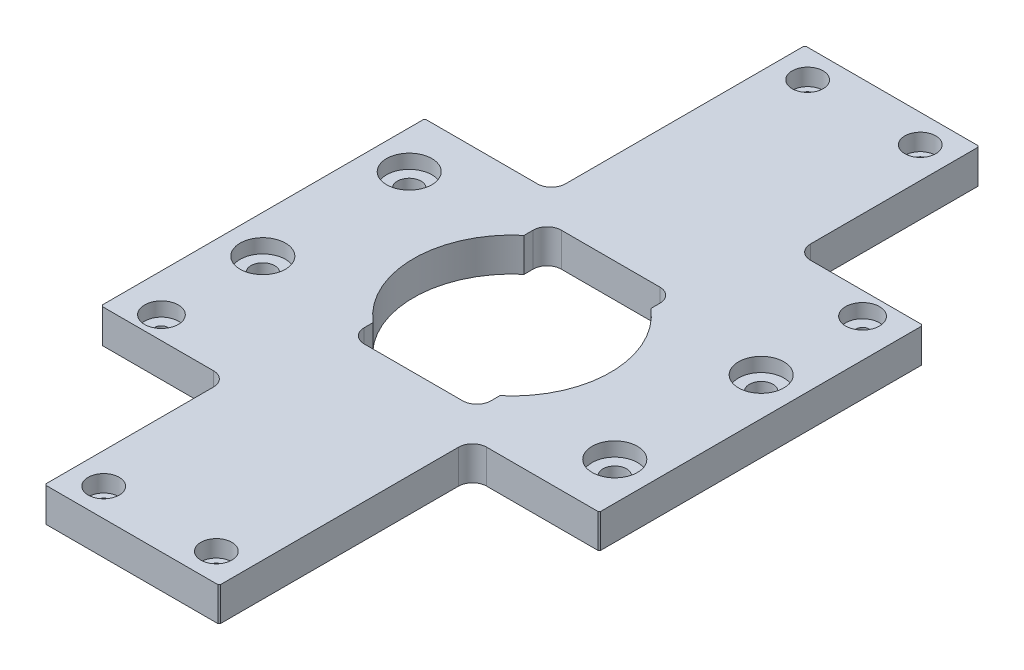
SolidWorks part; units mm, degrees
material "AL6061"
ref_plane "Front Plane" through (0, 0, 0) normal (0, 0, 1) x (1, 0, 0)
ref_plane "Top Plane" through (0, 0, 0) normal (0, 1, 0) x (1, 0, 0)
ref_plane "Right Plane" through (0, 0, 0) normal (1, 0, 0) x (0, 0, -1)
sketch "Sketch1" plane through (0, 0, 0) normal (0, 1, 0) x (1, 0, 0)
  line L1 (-76, -135) -> (76, -135)
  line L2 (-76, -135) -> (-76, 135)
  line L3 (-76, 135) -> (76, 135)
  line L4 (76, -135) -> (76, 135)
  line L5 (-76, -135) -> (76, 135) construction
  line L6 (-76, 135) -> (76, -135) construction
  point P0 (0, 0)
  dimension "D1" = 152
  dimension "D2" = 270
extrude "Boss-Extrude1" add sketch "Sketch1" along normal mid plane 12
sketch "Sketch2" plane through (0, 6, 0) normal (0, 1, 0) x (1, 0, 0)
  circle A0 centre (0, 0) radius 35
  dimension "D1" = 70
extrude "Cut-Extrude1" cut sketch "Sketch2" against normal through all
sketch "Sketch5" plane through (0, 6, 0) normal (0, 1, 0) x (1, 0, 0)
  line L0 (0, 0) -> (-109.7295, 0) construction
  line L1 (0, 0) -> (0, 145.3543) construction
  line L2 (62.5, 62) -> (62.5, -123.0833) construction
  circle A0 centre (62.5, 62) radius 6
  circle A1 centre (-62.5, 62) radius 6 construction
  circle A2 centre (-62.5, -62) radius 6
  circle A3 centre (62.5, -62) radius 6 construction
  circle A4 centre (62.5, 26) radius 8.05
  circle A5 centre (-62.5, 26) radius 8.05
  circle A6 centre (-62.5, -26) radius 8.05
  circle A7 centre (62.5, -26) radius 8.05
  dimension "D1" = 124
  dimension "D2" = 125
  dimension "D3" = 12
  dimension "D4" = 16.1
  dimension "D5" = 52
extrude "Cut-Extrude2" cut sketch "Sketch5" against normal blind 5
sketch "Sketch6" plane through (0, 6, 0) normal (0, 1, 0) x (1, 0, 0)
  line L1 (-22.5, -35) -> (22.5, -35)
  line L2 (-22.5, -35) -> (-22.5, 35)
  line L3 (-22.5, 35) -> (22.5, 35)
  line L4 (22.5, -35) -> (22.5, 35)
  line L5 (-22.5, -35) -> (22.5, 35) construction
  line L6 (-22.5, 35) -> (22.5, -35) construction
  point P0 (0, 0)
  dimension "D1" = 70
  dimension "D2" = 45
extrude "Cut-Extrude3" cut sketch "Sketch6" against normal through all
sketch "Sketch7" plane through (0, 6, 0) normal (0, 1, 0) x (1, 0, 0)
  line L0 (0, 0) -> (0, 159.161) construction
  line L1 (0, 0) -> (-111.7004, 0) construction
  line L2 (31, 135) -> (31, 45) construction
  line L3 (-76, 135) -> (-31, 135)
  line L4 (-76, 135) -> (-76, 45)
  line L5 (-76, 45) -> (-31, 45)
  line L6 (-31, 135) -> (-31, 45)
  line L7 (76, 45) -> (31, 45) construction
  line L8 (76, 135) -> (76, 45) construction
  line L9 (76, 135) -> (31, 135) construction
  line L10 (76, -135) -> (31, -135)
  line L11 (76, -135) -> (76, -45)
  line L12 (76, -45) -> (31, -45)
  line L13 (-31, -135) -> (-31, -45) construction
  line L14 (-76, -45) -> (-31, -45) construction
  line L15 (-76, -135) -> (-76, -45) construction
  line L16 (-76, -135) -> (-31, -135) construction
  line L17 (31, -135) -> (31, -45)
  dimension "D1" = 45
  dimension "D2" = 90
extrude "Cut-Extrude4" cut sketch "Sketch7" against normal through all
sketch "Sketch8" plane through (0, -6, 0) normal (0, -1, 0) x (1, 0, 0)
  line L0 (0, 0) -> (110.8614, 0) construction
  line L1 (0, 0) -> (0, 168.5573) construction
  line L3 (-76, 135) -> (31, 135) construction
  circle A2 centre (-20, 125) radius 7.5
  circle A3 centre (20, 125) radius 7.5
  circle A4 centre (20, -125) radius 7.5
  circle A5 centre (-20, -125) radius 7.5
  dimension "D1" = 15
  dimension "D2" = 10
  dimension "D3" = 40
extrude "Cut-Extrude5" cut sketch "Sketch8" against normal blind 2
sketch "Sketch9" plane through (0, -6, 0) normal (0, -1, 0) x (1, 0, 0)
  line L0 (0, 0) -> (0, 166.3831) construction
  line L1 (-76, 135) -> (-31, 135)
  line L2 (-76, 135) -> (-76, 70)
  line L3 (-76, 70) -> (-31, 70)
  line L4 (-31, 135) -> (-31, 70)
  line L5 (0, 0) -> (-188.5113, 0) construction
  line L6 (-31, -135) -> (-31, -70) construction
  line L7 (-76, -70) -> (-31, -70) construction
  line L8 (-76, -135) -> (-76, -70) construction
  line L9 (-76, -135) -> (-31, -135) construction
  line L10 (76, -135) -> (31, -135)
  line L11 (76, -135) -> (76, -70)
  line L12 (76, -70) -> (31, -70)
  line L13 (31, -135) -> (31, -70)
  dimension "D1" = 45
  dimension "D2" = 140
extrude "Cut-Extrude6" cut sketch "Sketch9" against normal through all
fillet "Fillet1" radius 5 8 edges at (-31, 0, 70) (31, 0, 45) (-31, 0, -45) (31, 0, -70) (22.5, 0, -35) (-22.5, 0, -35) (22.5, 0, 35) (-22.5, 0, 35)
hole_wizard "Hole size per socket head cap screw type 2" positions "Sketch10" profile "Sketch11" counterbore size "M6" standard "GB" end condition through all
sketch "Sketch10" plane through (0, 6, 0) normal (0, 1, 0) x (1, 0, 0)
  point P0 (-20, 125)
  point P3 (20, 125)
  point P6 (-20, -125)
  point P9 (20, -125)
sketch "Sketch11" plane through (-20, 6, -125) normal (1, 0, 0) x (0, 0, 1)
  line L0 (0, 0) -> (0, 12)
  line L1 (0, 12) -> (3.3, 12)
  line L3 (3.3, 12) -> (3.3, 6)
  line L4 (3.3, 6) -> (5.5, 6)
  line L5 (5.5, 6) -> (5.5, 0)
  line L7 (5.5, 0) -> (0, 0)
  line L11 (0, -6.35) -> (0, 107.95) construction
  dimension "通孔孔直径" = 6.6
  dimension "通孔孔深度" = 12
  dimension "柱形沉头孔直径" = 11
  dimension "柱形沉头孔深度" = 6
hole_wizard "打孔尺寸(%根据)内六角圆柱头螺钉的类型2" positions "Sketch12" profile "Sketch13" counterbore size "M4" standard "GB" end condition through all
sketch "Sketch12" plane through (0, -6, 0) normal (0, -1, 0) x (-1, 0, 0)
  point P0 (62.5, -62)
  point P3 (-62.5, 62)
sketch "Sketch13" plane through (-62.5, -6, 62) normal (1, 0, 0) x (0, 0, -1)
  line L0 (0, 0) -> (0, 12)
  line L1 (0, 12) -> (2.25, 12)
  line L3 (2.25, 12) -> (2.25, 4)
  line L4 (2.25, 4) -> (4, 4)
  line L5 (4, 4) -> (4, 0)
  line L7 (4, 0) -> (0, 0)
  line L11 (0, -6.35) -> (0, 107.95) construction
  dimension "通孔孔直径" = 4.5
  dimension "通孔孔深度" = 12
  dimension "柱形沉头孔直径" = 8
  dimension "柱形沉头孔深度" = 4
hole_wizard "M8 Clearance Hole1" positions "Sketch14" profile "Sketch15" hole size "M8" standard "GB" end condition through all
sketch "Sketch14" plane through (0, -6, 0) normal (0, -1, 0) x (-1, 0, 0)
  point P0 (62.5, -26)
  point P3 (62.5, 26)
  point P6 (-62.5, -26)
  point P9 (-62.5, 26)
sketch "Sketch15" plane through (-62.5, -6, 26) normal (1, 0, 0) x (0, 0, -1)
  line L0 (0, 0) -> (0, 12)
  line L1 (0, 12) -> (4.2, 12)
  line L2 (4.2, 12) -> (4.2, 0)
  line L5 (4.2, 0) -> (0, 0)
  line L11 (0, -6.35) -> (0, 107.95) construction
  dimension "通孔孔直径" = 8.4
  dimension "通孔孔深度" = 12
chamfer "Chamfer1" distance 0.5 angle 45 8 edges at (76, 0, 45) (31, 0, 135) (-31, 0, 135) (-76, 0, 70) (-76, 0, -45) (76, 0, -70) (31, 0, -135) (-31, 0, -135)
